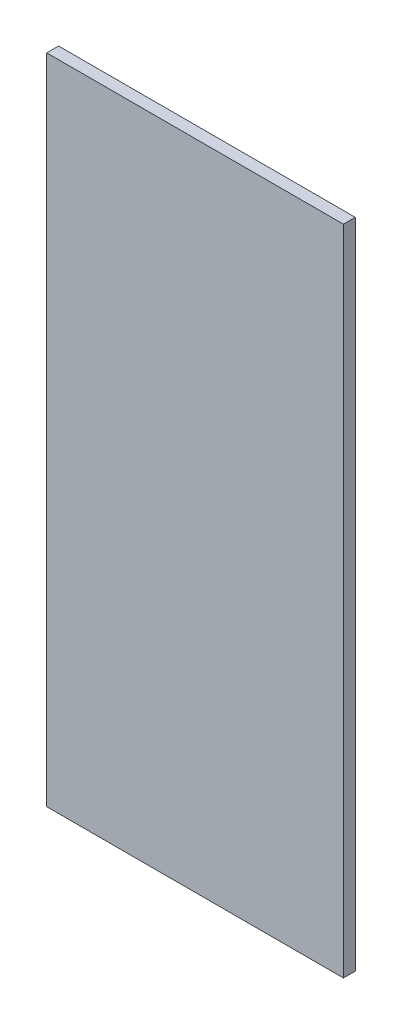
SolidWorks part; units mm, degrees
material "标准件"
ref_plane "前视基准面" through (0, 0, 0) normal (0, 0, 1) x (1, 0, 0)
ref_plane "上视基准面" through (0, 0, 0) normal (0, 1, 0) x (1, 0, 0)
ref_plane "右视基准面" through (0, 0, 0) normal (1, 0, 0) x (0, 0, -1)
sketch "草图1" plane through (0, 0, 0) normal (0, 0, 1) x (1, 0, 0)
  line L1 (-25, -55) -> (25, -55)
  line L2 (-25, -55) -> (-25, 55)
  line L3 (-25, 55) -> (25, 55)
  line L4 (25, -55) -> (25, 55)
  line L5 (-25, -55) -> (25, 55) construction
  line L6 (-25, 55) -> (25, -55) construction
  point P0 (0, 0)
  dimension "D1" = 50
  dimension "D2" = 110
extrude "凸台-拉伸1" add sketch "草图1" along normal mid plane 2
